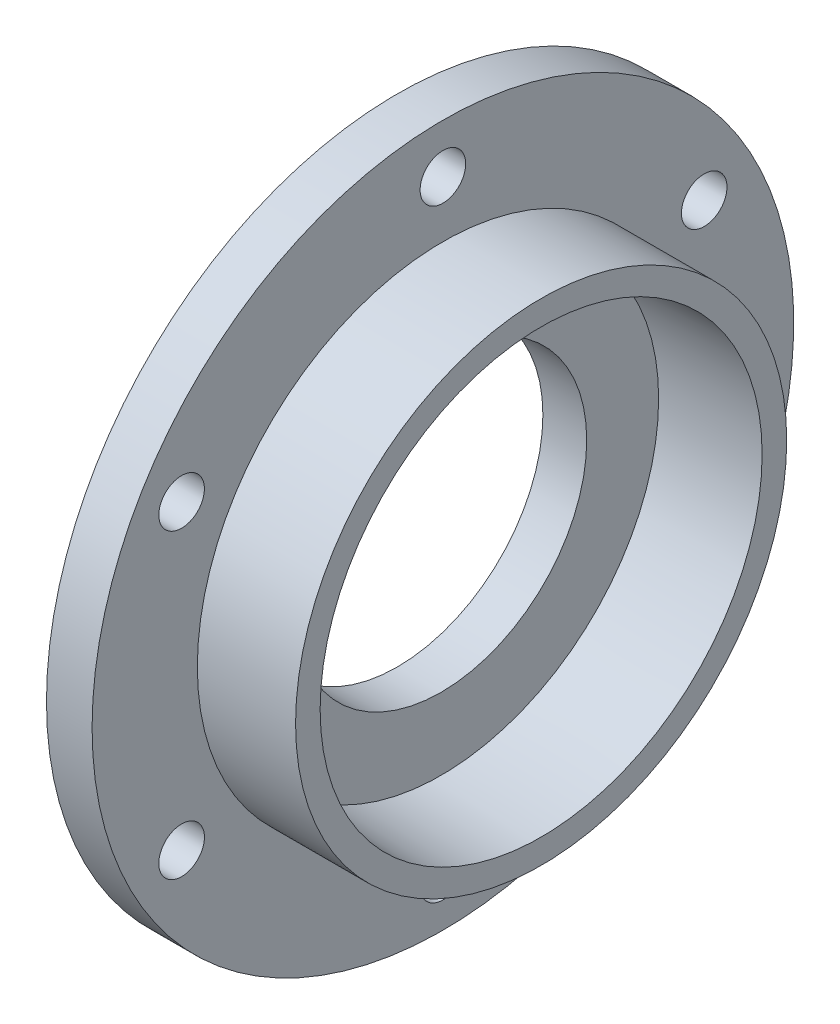
SolidWorks part; units mm, degrees
ref_plane "Front Plane" through (0, 0, 0) normal (0, 0, 1) x (1, 0, 0)
ref_plane "Top Plane" through (0, 0, 0) normal (0, 1, 0) x (1, 0, 0)
ref_plane "Right Plane" through (0, 0, 0) normal (1, 0, 0) x (0, 0, -1)
other "Configuration Table"
sketch "Sketch1" plane through (0, 0, 0) normal (0, 0, 1) x (1, 0, 0)
  line L0 (0, 0) -> (40.155, 0) construction
  line L1 (0, 0) -> (0, 100)
  line L2 (0, 100) -> (13, 100)
  line L3 (13, 100) -> (13, 70)
  line L4 (13, 70) -> (41, 70)
  line L5 (41, 70) -> (41, 62)
  line L6 (41, 62) -> (12.4952, 62)
  line L7 (12.4952, 62) -> (12.4952, 0)
  line L8 (12.4952, 0) -> (0, 0)
  dimension "D1" = 100
  dimension "D2" = 13
  dimension "D3" = 28
  dimension "D4" = 62
  dimension "D5" = 70
revolve "Revolve1" add sketch "Sketch1" angle 360 about L0
sketch "Sketch2" plane through (13, 0, 0) normal (1, 0, 0) x (0, 0, -1)
  line L0 (0, 0) -> (0, 106.2119) construction
  circle A0 centre (0, 0) radius 86 construction
  circle A1 centre (0, 86) radius 6.5
  dimension "D1" = 172
  dimension "D2" = 13
extrude "Cut-Extrude1" cut sketch "Sketch2" against normal through all
pattern_circular "CirPattern1" count 6 over 360 about axis through (0, 0, 0) along (1, 0, 0) of "Cut-Extrude1"
sketch "Sketch3" plane through (0, 0, 0) normal (-1, 0, 0) x (0, 0, 1)
  circle A0 centre (0, 0) radius 41.5
  dimension "D1" = 83
extrude "Cut-Extrude2" cut sketch "Sketch3" against normal through all
draft "Draft1" type of draft neutral plane draft angle 2 faces to draft 1 face at (41, 0, 62) neutral plane through (12.4952, 62, 0) neutral plane normal (1, 0, 0) parameters "D1"=2
